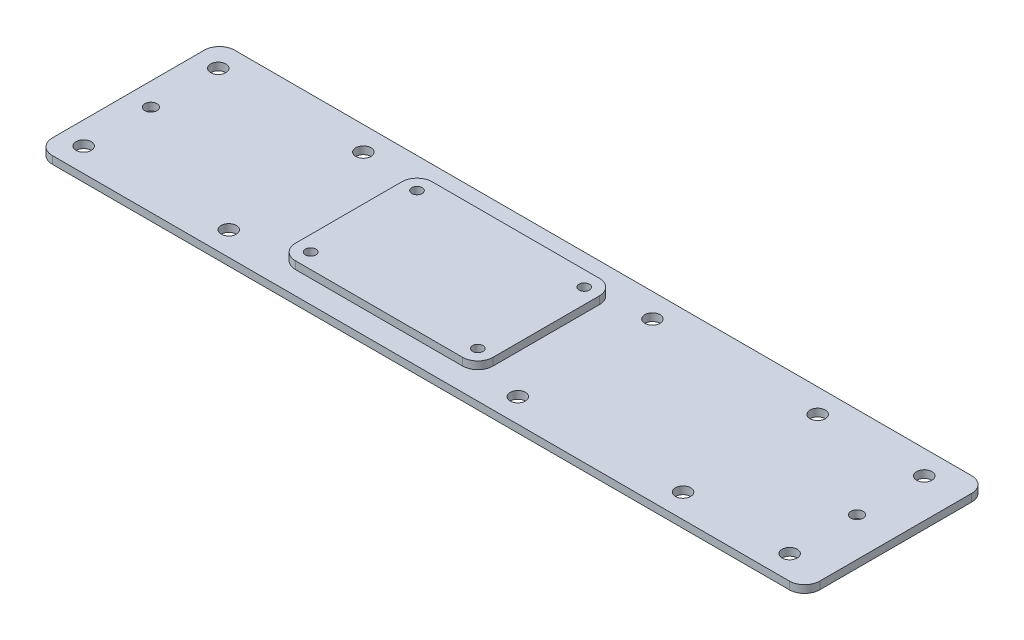
SolidWorks part; units mm, degrees
ref_plane "Front Plane" through (0, 0, 0) normal (0, 0, 1) x (1, 0, 0)
ref_plane "Top Plane" through (0, 0, 0) normal (0, 1, 0) x (1, 0, 0)
ref_plane "Right Plane" through (0, 0, 0) normal (1, 0, 0) x (0, 0, -1)
other "Configuration Table"
sketch "Sketch1" plane through (0, 539, 0) normal (0, 1, 0) x (1, 0, 0)
  line L0 (529, 129.05) -> (326.3063, 129.05) construction
  line L1 (-210, 69.05) -> (295, 69.05)
  line L2 (-210, 69.05) -> (-210, 189.05)
  line L3 (-210, 189.05) -> (295, 189.05)
  line L4 (295, 69.05) -> (295, 189.05)
  line L5 (529, 205) -> (529, 53.1) construction
  line L6 (0, 0) -> (0, -162.0008) construction
  line L8 (-50, 159.05) -> (50, 159.05)
  line L9 (-50, 159.05) -> (-50, 99.05)
  line L10 (-50, 99.05) -> (50, 99.05)
  line L11 (50, 159.05) -> (50, 99.05)
  dimension "D1" = 505
  dimension "D2" = 120
  dimension "D3" = 210
  dimension "D4" = 60
  dimension "D5" = 100
  dimension "D6" = 30
  dimension "D7" = 50
extrude "Boss-Extrude1" add sketch "Sketch1" along normal blind 5
fillet "Fillet1" radius 10 4 edges at (-210, 541.5, -69.05) (-210, 541.5, -189.05) (295, 541.5, -69.05) (295, 541.5, -189.05)
fillet "Fillet2" radius 10 4 edges at (50, 541.5, -99.05) (-50, 541.5, -99.05) (-50, 541.5, -159.05) (50, 541.5, -159.05)
sketch "Sketch2" plane through (0, 544, 0) normal (0, 1, 0) x (1, 0, 0)
  line L0 (40, 159.05) -> (-40, 159.05) construction
  line L1 (-55, 174.05) -> (55, 174.05)
  line L2 (-65, 164.05) -> (-65, 94.05)
  line L3 (-55, 84.05) -> (55, 84.05)
  line L4 (65, 164.05) -> (65, 94.05)
  line L5 (-40, 99.05) -> (40, 99.05) construction
  line L6 (50, 109.05) -> (50, 149.05) construction
  line L7 (-50, 149.05) -> (-50, 109.05) construction
  arc A0 (55, 174.05) -> (65, 164.05) centre (55, 164.05) cw
  arc A1 (-65, 94.05) -> (-55, 84.05) centre (-55, 94.05) ccw
  arc A2 (55, 84.05) -> (65, 94.05) centre (55, 94.05) ccw
  arc A3 (-55, 174.05) -> (-65, 164.05) centre (-55, 164.05) ccw
  dimension "D5" = 10
  dimension "D1" = 15
  dimension "D2" = 15
  dimension "D3" = 15
  dimension "D4" = 15
extrude "Boss-Extrude2" add sketch "Sketch2" along normal blind 5 separate body
hole_wizard "M8 Tapped Hole1" positions "Sketch3" profile "Sketch4" tap size "M8" standard "GB"
sketch "Sketch3" plane through (0, 549, 0) normal (0, 1, 0) x (1, 0, 0)
  point P0 (-55, 164.05)
  point P3 (55, 164.05)
  point P6 (-55, 94.05)
  point P9 (55, 94.05)
sketch "Sketch4" plane through (-55, 549, -164.05) normal (1, 0, 0) x (0, 0, 1)
  line L0 (0, 0) -> (0, 22.25)
  line L1 (0, 22.25) -> (3.4, 20.2071)
  line L2 (3.4, 20.2071) -> (3.4, 0)
  line L5 (3.4, 0) -> (0, 0)
  line L10 (0, 22.25) -> (-3.4, 20.2071) construction
  line L11 (0, -6.35) -> (0, 107.95) construction
  dimension "螺纹孔钻头直径" = 6.8
  dimension "螺纹孔钻头深度" = 22.25
  dimension "导头角度" = 118
cosmetic thread "Cosmetic Thread1" parameters "D1"=16, "D2"=8
cosmetic thread "Cosmetic Thread2" parameters "D1"=16, "D2"=8
cosmetic thread "Cosmetic Thread3" parameters "D1"=16, "D2"=8
cosmetic thread "Cosmetic Thread4" parameters "D1"=16, "D2"=8
sketch "Sketch5" plane through (0, 544, 0) normal (0, 1, 0) x (1, 0, 0)
  line L0 (295, 129.05) -> (356.5066, 129.05) construction
  line L1 (295, 79.05) -> (295, 179.05) construction
  line L2 (-659.5984, 173.3318) -> (269.4766, 173.3318) construction
  circle A0 centre (-195.0609, 173.3318) radius 5
  circle A1 centre (-99.5785, 173.3318) radius 5
  circle A2 centre (90.6254, 173.3318) radius 5
  circle A3 centre (199.333, 173.3318) radius 5
  circle A4 centre (269.4766, 173.3318) radius 5
  circle A5 centre (269.4766, 129.05) radius 4
  circle A6 centre (-195.0609, 129.05) radius 4
  circle A7 centre (269.4766, 84.7682) radius 5
  circle A8 centre (199.333, 84.7682) radius 5
  circle A9 centre (90.6254, 84.7682) radius 5
  circle A10 centre (-99.5785, 84.7682) radius 5
  circle A11 centre (-195.0609, 84.7682) radius 5
  point P21 (-195.0609, 173.3318)
  dimension "D1" = 10
  dimension "D2" = 95.4823
  dimension "D3" = 8
  dimension "D4" = 8
extrude "Cut-Extrude1" cut sketch "Sketch5" against normal blind 20
